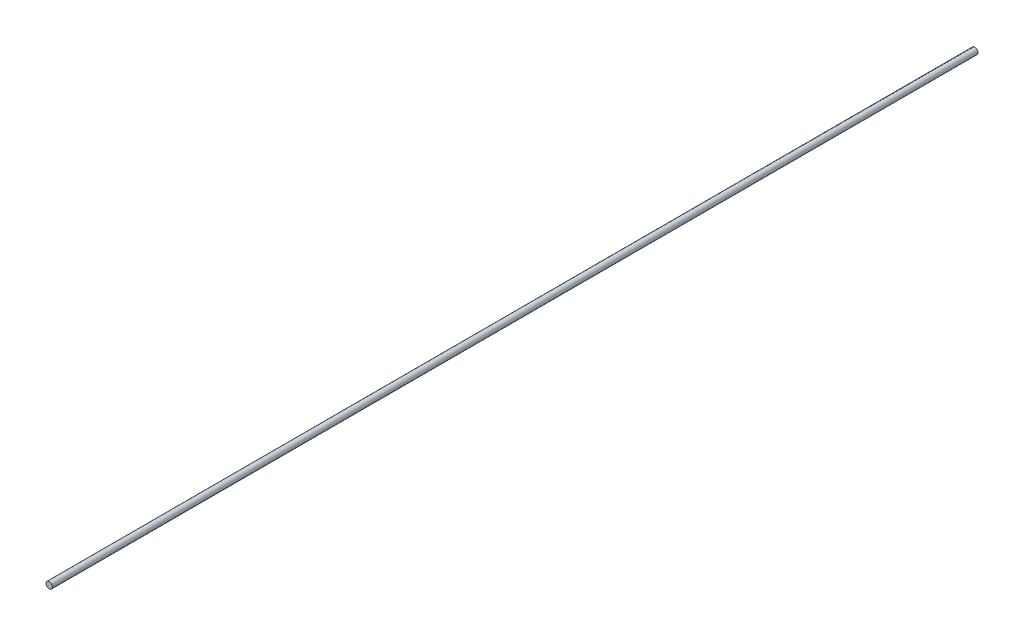
SolidWorks part; units mm, degrees
material "SWM-B"
ref_plane "Front Plane" through (0, 0, 0) normal (0, 0, 1) x (1, 0, 0)
ref_plane "Top Plane" through (0, 0, 0) normal (0, 1, 0) x (1, 0, 0)
ref_plane "Right Plane" through (0, 0, 0) normal (1, 0, 0) x (0, 0, -1)
sketch "Sketch1" plane through (0, 0, 0) normal (0, 0, 1) x (1, 0, 0)
  circle A0 centre (0, 0) radius 3
  dimension "D1" = 6
extrude "Boss-Extrude1" add sketch "Sketch1" along normal blind 875
